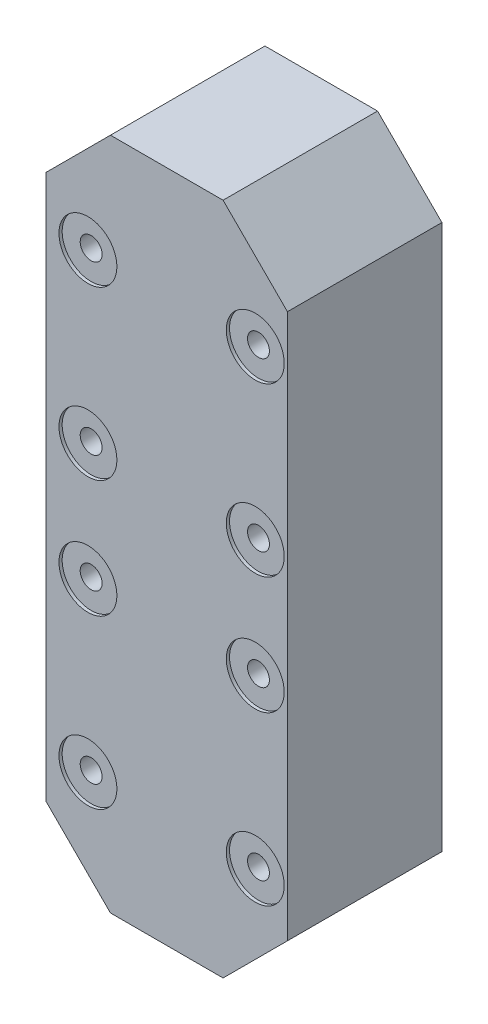
from build123d import *

# Parameters (mm, degrees)
BOSS_EXTRUDE1_DEPTH                     = 24
BOSS_EXTRUDE1_DEPTH_BACK                = 2
SKETCH1_W                               = 37.5
SKETCH1_H                               = 104.65705171
SKETCH2_W                               = 35
SKETCH2_H                               = 2
CUT_EXTRUDE1_DEPTH                      = 110.129961388
CHAMFER1_SIZE                           = 10
CBORE_FOR_M3_HEX_HEAD_BOLT1_D           = 3.4
CBORE_FOR_M3_HEX_HEAD_BOLT1_CBORE_D     = 9
CBORE_FOR_M3_HEX_HEAD_BOLT1_CBORE_DEPTH = 0.5


with BuildPart() as part:
    # Sketch1 → Boss-Extrude1 (new, two sides: drawn at the far end of the back side and taken through both)
    with BuildSketch(Plane.XY.offset(-BOSS_EXTRUDE1_DEPTH_BACK)):
        with Locations((-0.75, -2.428525855)):
            Rectangle(SKETCH1_W, SKETCH1_H)
    extrude(amount=BOSS_EXTRUDE1_DEPTH + BOSS_EXTRUDE1_DEPTH_BACK)

    # Sketch2 → Cut-Extrude1 (cut, through all)
    with BuildSketch(Plane.XZ.offset(54.75705171)):
        with Locations((0.5, -1)):
            Rectangle(SKETCH2_W, SKETCH2_H)
    extrude(amount=-CUT_EXTRUDE1_DEPTH, mode=Mode.SUBTRACT)

    # Chamfer1
    chamfer1_edges = [part.edges().sort_by_distance(p)[0] for p in [
        (18, -54.75705171, 12),
        (-19.5, -54.75705171, 11),
        (18, 49.9, 12),
        (-19.5, 49.9, 11),
    ]]
    chamfer(chamfer1_edges, length=CHAMFER1_SIZE)

    # CBORE for M3 Hex Head Bolt1 (through all)
    with Locations(Plane.XY.offset(24)):
        with Locations((-13, 32.7), (13, 32.7), (13, 6.7), (-13, 6.7), (-13, -11.55705171), (13, -11.55705171), (13, -37.55705171), (-13, -37.55705171)):
            CounterBoreHole(CBORE_FOR_M3_HEX_HEAD_BOLT1_D / 2, CBORE_FOR_M3_HEX_HEAD_BOLT1_CBORE_D / 2, CBORE_FOR_M3_HEX_HEAD_BOLT1_CBORE_DEPTH)


solid = part.part
